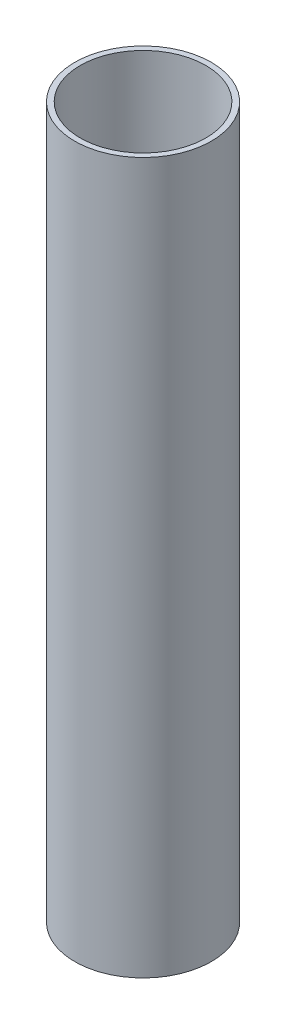
SolidWorks part; units mm, degrees
material "铜H591"
ref_plane "前视基准面" through (0, 0, 0) normal (0, 0, 1) x (1, 0, 0)
ref_plane "上视基准面" through (0, 0, 0) normal (0, 1, 0) x (1, 0, 0)
ref_plane "右视基准面" through (0, 0, 0) normal (1, 0, 0) x (0, 0, -1)
sketch "草图1" plane through (0, 0, 0) normal (0, 1, 0) x (1, 0, 0)
  circle A0 centre (0, 0) radius 2.5
  circle A1 centre (0, 0) radius 2.3
  dimension "D1" = 5
  dimension "D2" = 4.6
extrude "凸台-拉伸1" add sketch "草图1" along normal blind 26
